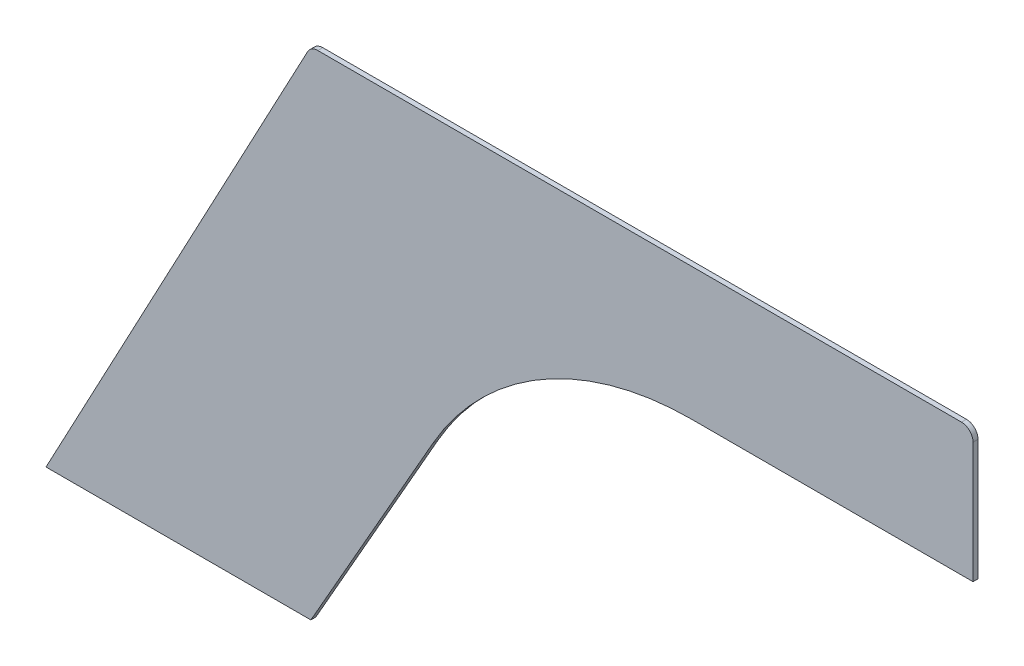
from build123d import *

# Parameters (mm, degrees)
BOSS_EXTRUDE1_DEPTH = 1.5


with BuildPart() as part:
    # Sketch1 → Boss-Extrude1 (new body)
    with BuildSketch(Plane.XY):
        with BuildLine():
            Line((0, 0), (79.011764706, 148.147058824))
            ThreePointArc((79.011764706, 148.147058824), (80.299264856, 149.50122524), (82.1, 150))
            Line((82.1, 150), (276.5, 150))
            ThreePointArc((276.5, 150), (278.974873734, 148.974873734), (280, 146.5))
            Line((280, 146.5), (280, 110))
            Line((280, 110), (195, 110))
            ThreePointArc((195, 110), (149.787439916, 97.819177653), (116.813238993, 64.573875793))
            Line((116.813238993, 64.573875793), (80, 0))
            Line((80, 0), (0, 0))
        make_face()
    extrude(amount=BOSS_EXTRUDE1_DEPTH)


solid = part.part
